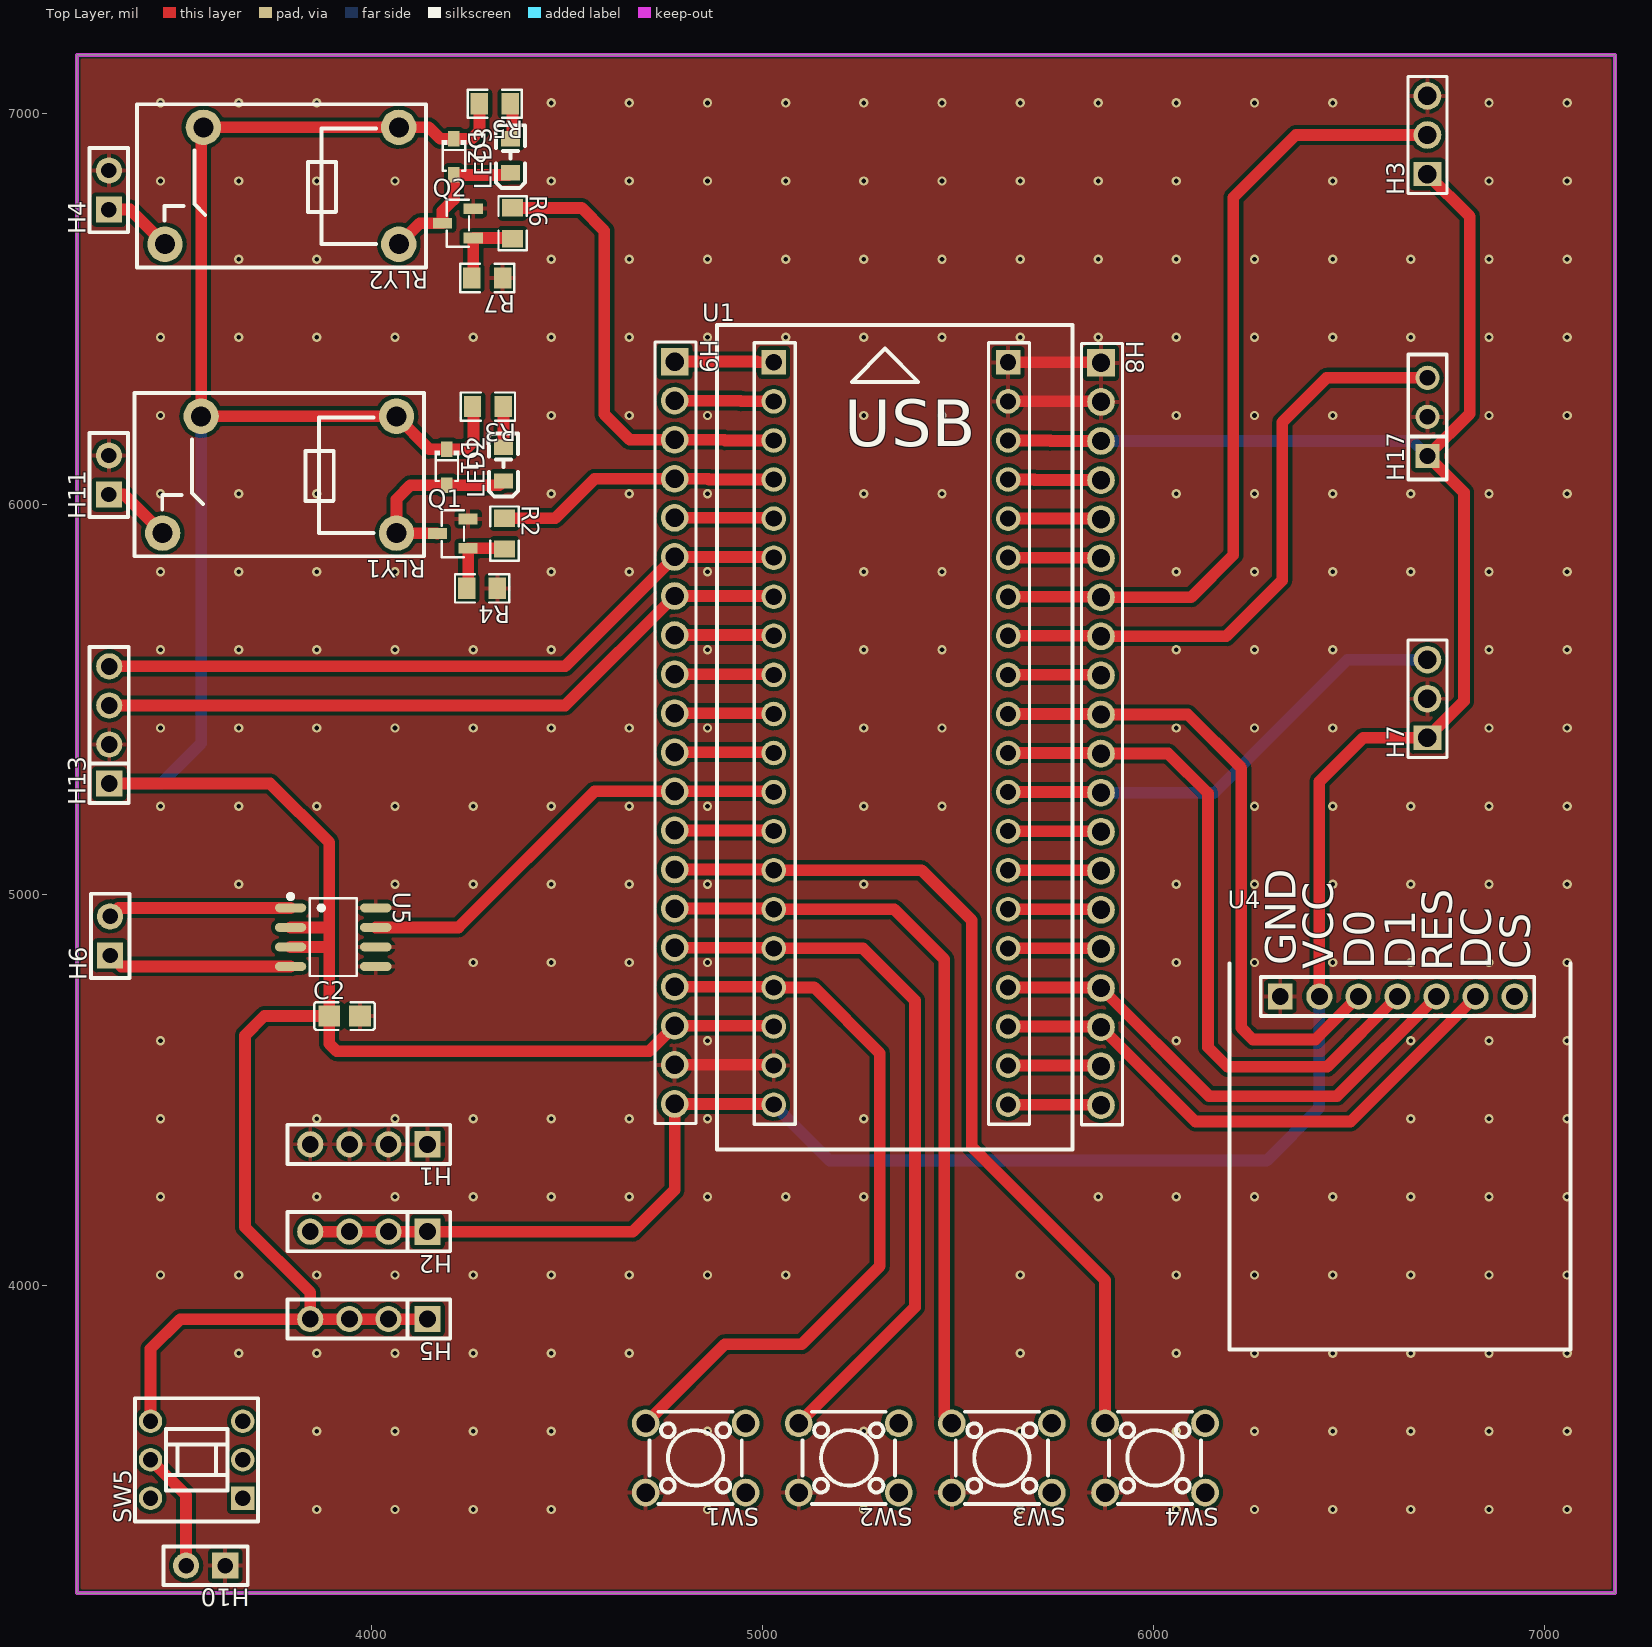
[diagram p0: Top Layer view]
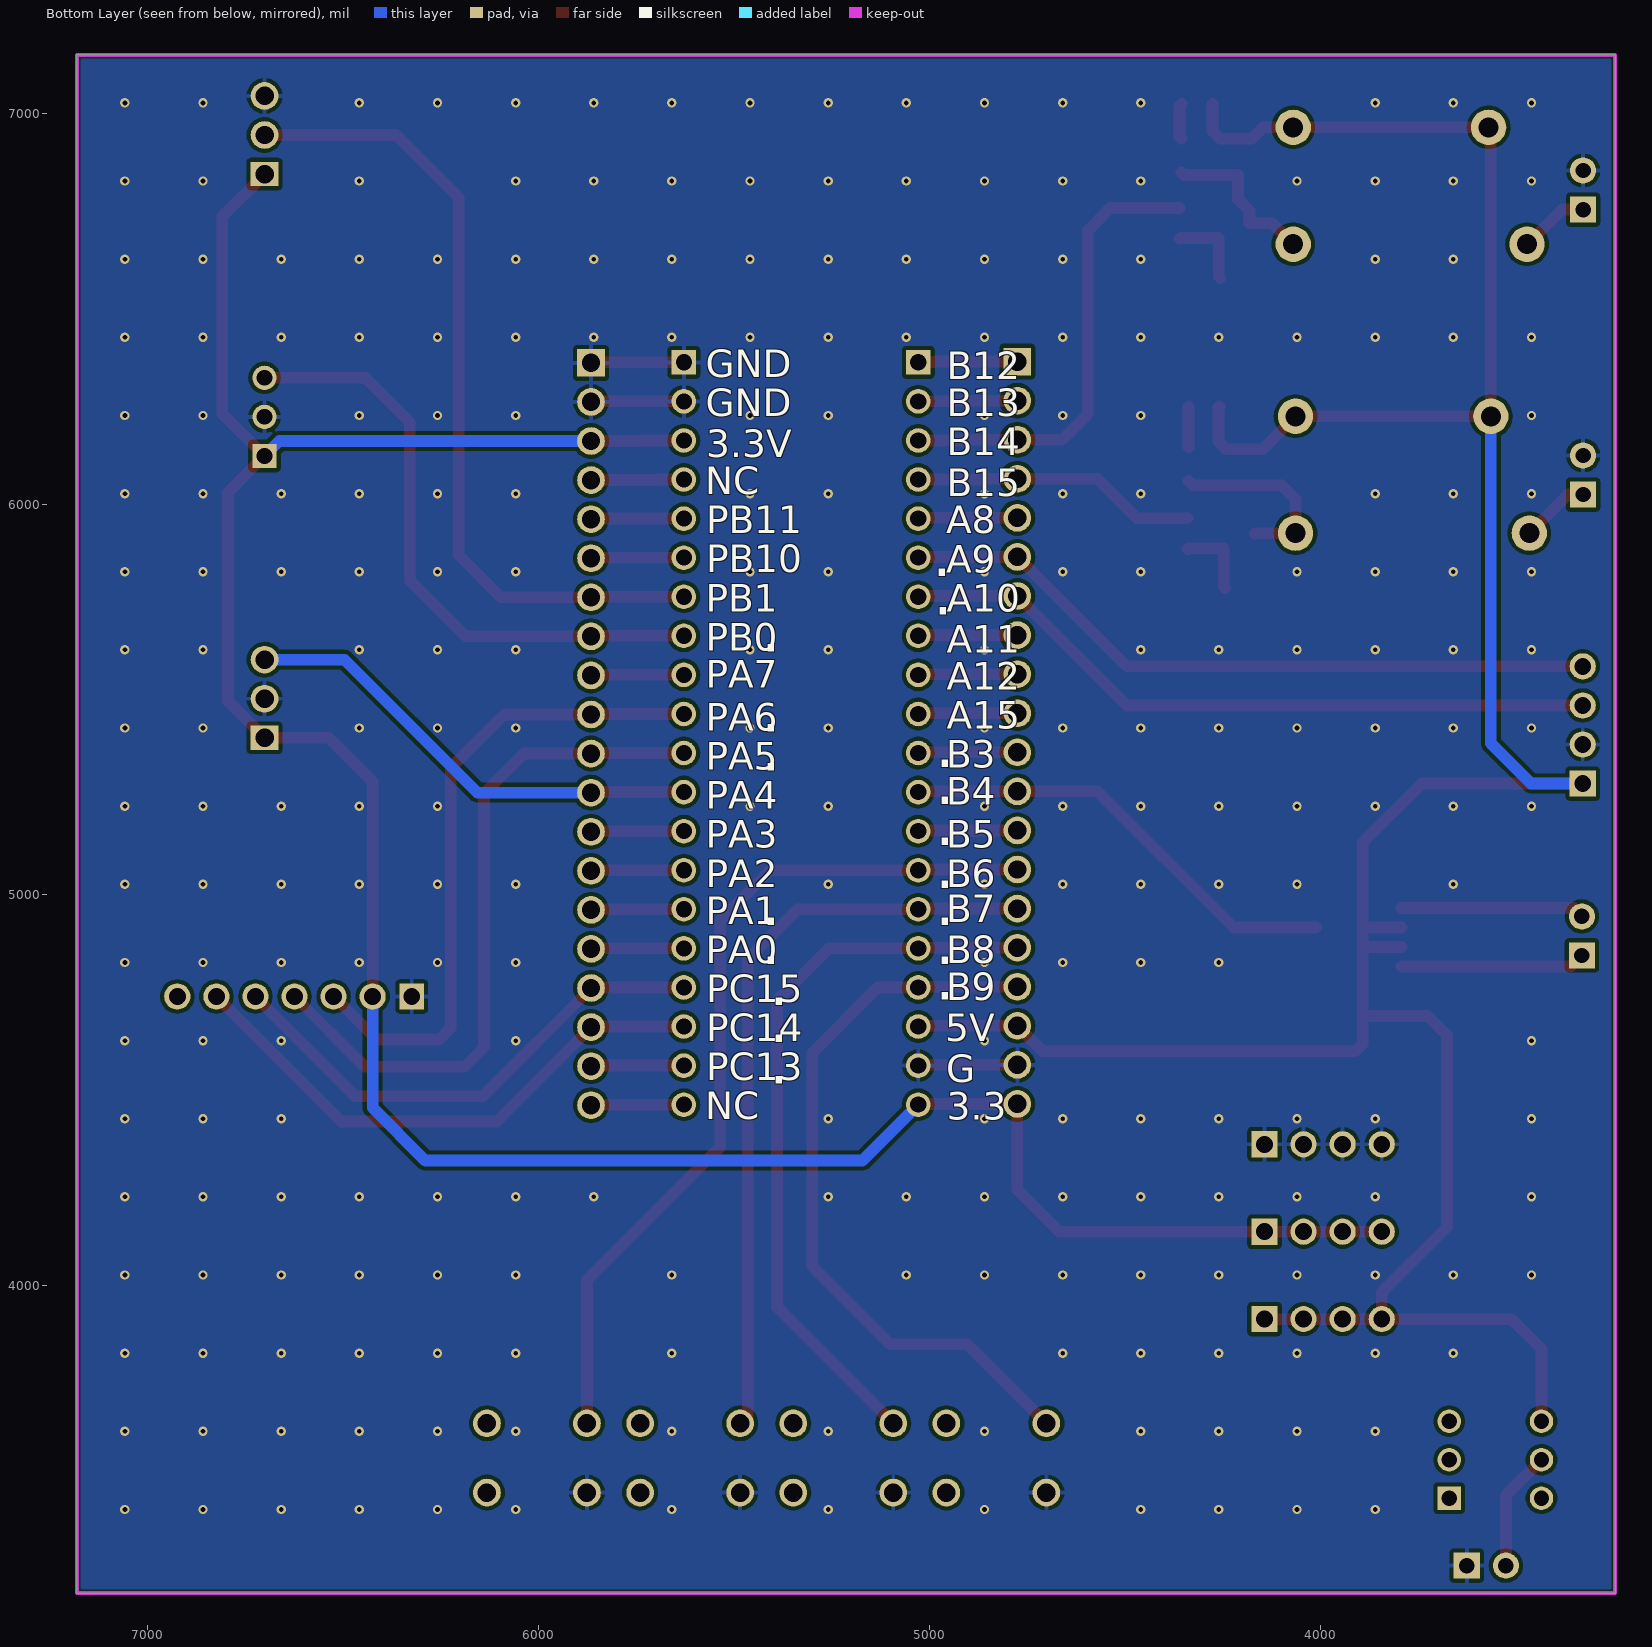
[diagram p1: Bottom Layer view, seen from below]
# Altium PCB MISC51992.pcbdoc
Units mil, origin at the board's own origin, x right, y up, seen from the top; angles counter-clockwise.
Board outline 3937.01 x 3937.01 mil, 2 copper layers (Top Layer, Bottom Layer), stack 62.206 mil thick; 36 components, 48 nets, 186 pads, 262 vias.

## Layer stack, top to bottom
Top Solder Mask Layer: solder mask 0.394, Dk 3.3
Top Layer: signal copper 1.379
Dielectric1: surface 59.449, FR4, Dk 4.5
Bottom Layer: signal copper 1.378
Bottom Solder Mask Layer: solder mask 0.394, Dk 3.3

## Board outline
3245,7150 3245,3212.99 7182.01,3212.99 7182.01,7150

## Design rules (kind name [scope] priority, off if disabled: settings)
BoardOutlineClearance copperThickness2oz_1 [All] p2 off: genericclearance=7.99 ignorepadtopadclearanceinfootprint=FALSE except(0: Arc-SplitContinuation Track-SplitContinuation SMDPad-SplitContinuation THPad-SplitContinuation Via-SplitContinuation Fill-SplitContinuation Region-SplitContinuation Poly-SplitContinuation Text-SplitContinuation Hole-SplitContinuation; 5.98: Arc-CutoutEdge SMDPad-CutoutEdge THPad-CutoutEdge Via-CutoutEdge Fill-CutoutEdge Region-CutoutEdge Text-CutoutEdge; 6.93: Hole-OutlineEdge Hole-CutoutEdge; 10: Poly-OutlineEdge Poly-CutoutEdge; 11.81: Arc-OutlineEdge Track-OutlineEdge SMDPad-OutlineEdge THPad-OutlineEdge Via-OutlineEdge Fill-OutlineEdge Region-OutlineEdge Text-OutlineEdge Track-CutoutEdge)
BoardOutlineClearance copperThickness1oz_1 [All] p4: genericclearance=4.02 ignorepadtopadclearanceinfootprint=FALSE except(0: Arc-SplitContinuation Track-SplitContinuation SMDPad-SplitContinuation THPad-SplitContinuation Via-SplitContinuation Fill-SplitContinuation Region-SplitContinuation Poly-SplitContinuation Text-SplitContinuation Hole-SplitContinuation; 6: SMDPad-CutoutEdge THPad-CutoutEdge Via-CutoutEdge Fill-CutoutEdge Region-CutoutEdge Text-CutoutEdge; 6.93: Hole-OutlineEdge Hole-CutoutEdge; 10: Poly-OutlineEdge Poly-CutoutEdge; 11.8: Arc-OutlineEdge Track-OutlineEdge SMDPad-OutlineEdge THPad-OutlineEdge Via-OutlineEdge Fill-OutlineEdge Region-OutlineEdge Text-OutlineEdge; 11.81: Arc-CutoutEdge Track-CutoutEdge)
Clearance copperThickness2oz [All] p1 off: gap=7.99 ignorepadtopadclearanceinfootprint=FALSE except(5.98: SMDPad-Track SMDPad-SMDPad THPad-Track SMDPad-THPad THPad-THPad Track-Via SMDPad-Via THPad-Via Via-Via Fill-Track Region-Track Fill-SMDPad Region-SMDPad Fill-THPad Region-THPad Fill-Via Region-Via Fill-Fill Fill-Region Region-Region Arc-Track Arc-SMDPad Arc-THPad Arc-Via Fill-Arc Region-Arc Arc-Arc Text-Track SMDPad-Text Text-THPad Text-Via Fill-Text Region-Text Arc-Text Text-Text; 6.93: Hole-Track Hole-SMDPad Hole-THPad Hole-Via Fill-Hole Region-Hole Hole-Arc Hole-Text; 10: Poly-Track Poly-SMDPad Poly-THPad Poly-Via Poly-Fill Poly-Region Poly-Poly Poly-Arc Poly-Text Poly-Hole)
Clearance copperThickness1oz [All] p3: gap=4.02 ignorepadtopadclearanceinfootprint=FALSE except(5.98: SMDPad-Track SMDPad-SMDPad THPad-Track SMDPad-THPad THPad-THPad Track-Via SMDPad-Via THPad-Via Via-Via Fill-Track Region-Track Fill-SMDPad Region-SMDPad Fill-THPad Region-THPad Fill-Via Region-Via Fill-Fill Fill-Region Region-Region; 6: Arc-Track Arc-SMDPad Arc-THPad Arc-Via Fill-Arc Region-Arc Arc-Arc Text-Track SMDPad-Text Text-THPad Text-Via Fill-Text Region-Text Arc-Text Text-Text; 6.93: Hole-Track Hole-SMDPad Hole-THPad Hole-Via Fill-Hole Region-Hole Hole-Arc Hole-Text; 10: Poly-Track Poly-SMDPad Poly-THPad Poly-Via Poly-Fill Poly-Region Poly-Poly Poly-Arc Poly-Text Poly-Hole)
DiffPairsRouting differentialPair [All] p1: maxlimit=6 minlimit=6 mostfreqgap=6 toplayer_minwidth=5 toplayer_prefwidth=10 toplayer_maxwidth=100 toplayer_mingap=6 toplayer_prefgap=6 toplayer_maxgap=6 bottomlayer_minwidth=5 bottomlayer_prefwidth=10 bottomlayer_maxwidth=100 bottomlayer_mingap=6 bottomlayer_prefgap=6 bottomlayer_maxgap=6 maxuncoupledlength=10
HoleToHoleClearance otherClearance [All] p1: gap=11.81 allowstackedmicrovias=TRUE
Length netLength [All] p1: minlimit=0 maxlimit=0
MatchedLengths netLengthTolerance [All] p1: tolerance=1000
PasteMaskExpansion pasteMaskExpansion [All] p1: expansion=0
PlaneConnect innerPlane [All] p1: planeconnectstyle=Relief reliefexpansion=20 reliefentries=4 reliefconductorwidth=10 reliefairgap=10
PolygonConnect copperRegion [(InNet('GND'))] p1: connectstyle=Relief reliefconductorwidth=10 reliefentries=4 polygonreliefangle="90 Angle" airgapwidth=10 via.connectstyle=Relief via.reliefconductorwidth=10 via.reliefentries=4 via.polygonreliefangle="90 Angle" via.airgapwidth=10
RoutingVias viaSize [All] p1: holewidth=12.01 width=24.02 viastyle="Through Hole" minholewidth=11.81 minwidth=19.68 maxholewidth=248.03 maxwidth=393.7
SolderMaskExpansion solderMaskExpansion [IsVia] p1: expansion=-1000 istentingtop=TRUE
SolderMaskExpansion solderMaskExpansion [All] p2: expansion=2 istentingtop=FALSE
Width copperThickness2oz_2 [All] p1 off: maxlimit=100 minlimit=8 preferedwidth=10
Width copperThickness1oz_2 [All] p2: maxlimit=100 minlimit=5 preferedwidth=10

## Components (designator, comment, footprint, x,y, rotation, side; value= is the part's Value field where it differs from the comment)
C2 "1uf" C0805 3930,4690 r0 top
D1 "1N4007WS" SOD-323_L1.8-W1.3-LS2.5-RD 4192.01,6094.72 r270 top
D2 "1N4007WS" SOD-323_L1.8-W1.3-LS2.5-RD 4210.11,6889 r270 top
H1 "" HDR-TH_4P-P2.54-V-F 3992.33,4361.73 r180 top
H2 "" HDR-TH_4P-P2.54-V-F 3992.33,4138.01 r180 top
H3 "Header-Male-2.54_1x3" HDR-TH_3P-P2.54-V-M-1 6701.59,6945 r90 top
H4 "" HDR-TH_2P-P2.54-V-F 3327.01,6804 r90 top
H5 "" HDR-TH_4P-P2.54-V-F 3992.33,3914.29 r180 top
H6 "" HDR-TH_2P-P2.54-V-F 3330,4895 r90 top
H7 "Header-Male-2.54_1x3" HDR-TH_3P-P2.54-V-M-1 6701.59,5502.04 r90 top
H8 "" HDR-TH_20P-P2.54-V-M-1 5866.11,5411.72 r270 top
H9 "" HDR-TH_20P-P2.54-V-M-1 4775,5415 r270 top
H10 "" HDR-TH_2P-P2.54-V-F 3574.54,3283.39 r180 top
H11 "" HDR-TH_2P-P2.54-V-F 3327.01,6074.72 r90 top
H13 "Header-Male-2.54_1x4" HDR-TH_4P-P2.54-V-M 3327.8,5435 r90 top
H17 "" HDR-TH_3P-P2.54-V-F 6701.81,6223.52 r90 top
LED2 "" LED_0805 4337.01,6104.72 r90 top
LED3 "" LED_0805 4355.11,6894 r90 top
Q1 "SS8050_C2150" SOT-23-3_L2.9-W1.3-P1.90-LS2.4-BR 4207.01,5924.72 r0 top
Q2 "SS8050_C2150" SOT-23-3_L2.9-W1.3-P1.90-LS2.4-BR 4220.11,6719 r0 top
R2 "4.7kΩ" R0805 4339.4,5924.81 r270 top
R3 "4.7kΩ" R0805 4297.01,6249.72 r180 top
R4 "10k" R0805 4282.01,5784.72 r180 top
R5 "4.7kΩ" R0805 4314.59,7025 r180 top
R6 "4.7kΩ" R0805 4360.11,6719 r270 top
R7 "10k" R0805 4295.11,6579 r180 top
RLY1 "JZC-32F/005-HS3(555)" RELAY-TH_JZC-32F-XXXHXX 3763.77,6075.44 r180 top
RLY2 "JZC-32F/005-HS3(555)" RELAY-TH_JZC-32F-XXXHXX 3769.59,6815 r180 top
SW1 "TS665CJ" SW-TH_4P-L6.0-W6.0-P4.50-LS6.5 4828.6,3558.98 r180 top
SW2 "TS665CJ" SW-TH_4P-L6.0-W6.0-P4.50-LS6.5 5220.56,3558.98 r180 top
SW3 "TS665CJ" SW-TH_4P-L6.0-W6.0-P4.50-LS6.5 5612.51,3558.98 r180 top
SW4 "TS665CJ" SW-TH_4P-L6.0-W6.0-P4.50-LS6.5 6004.47,3558.98 r180 top
SW5 "XKB8080-Z" SW-TH_6P-L8.0-W8.0-P2.50 3551.58,3554.25 r90 top
U1 "" STM32最小系统 5028.53,6363.15 r0 top
U4 "" OLED12864/7针 6325,4740 r0 top
U5 "L9110S_C2895059" SOP-8_L5.0-W4.0-P1.27-LS6.0-BL 3900.97,4891.78 r270 top

## Footprints (in the part's own frame and the unit in brackets; to place one, negate y for a bottom-side part, rotate by r counter-clockwise, add the part's x,y. Pads: shape width x height; smd on the part's side, far side on the other; paste and mask are expansions set on the pad)
C0805 [mm]
  rect 1.41x1.35 smd paste-100 mask+0.051: 1(-1,0) 2(1,0)
  silkscreen extent -1.96,-0.9 1.96,0.9
HDR-TH_2P-P2.54-V-F [mm]
  rect 1.7x1.7 hole 1: 1(-1.27,0)
  round 1.7 hole 1: 2(1.27,0)
  silkscreen extent -2.74,-1.25 2.74,1.25
HDR-TH_3P-P2.54-V-F [mil]
  rect 62x62 hole 40.16: 1(-100,0)
  round 62 hole 40.16: 2(0,0) 3(100,0)
  silkscreen extent -160,-49 160,49
HDR-TH_3P-P2.54-V-M-1 [mm]
  rect 1.575x1.8 hole 1.2: 1(-2.54,0)
  round 1.8 hole 1.2: 2(0,0) 3(2.54,0)
  silkscreen extent -3.81,-1.27 3.81,1.27
HDR-TH_4P-P2.54-V-F [mm]
  rect 1.7x1.7 hole 1.1: 1(-3.81,0)
  round 1.7 hole 1.1: 2(-1.27,0) 3(1.27,0) 4(3.81,0)
  silkscreen extent -5.29,-1.27 5.29,1.27
HDR-TH_4P-P2.54-V-M [mm]
  rect 1.7x1.7 hole 1.1: 1(-3.81,0)
  round 1.7 hole 1.1: 2(-1.27,0) 3(1.27,0) 4(3.81,0)
  silkscreen extent -5.08,-1.27 5.08,1.27
HDR-TH_20P-P2.54-V-M-1 [mm]
  rect 1.8x1.8 hole 1.2: 1(-24.13,0)
  round 1.8 hole 1.2: 2(-21.59,0) 3(-19.05,0) 4(-16.51,0) 5(-13.97,0) 6(-11.43,0) 7(-8.89,0) 8(-6.35,0) 9(-3.81,0) 10(-1.27,0) 11(1.27,0) 12(3.81,0) 13(6.35,0) 14(8.89,0) 15(11.43,0) 16(13.97,0) 17(16.51,0) 18(19.05,0) 19(21.59,0) 20(24.13,0)
  silkscreen extent -25.4,-1.27 25.4,1.4
LED_0805 [mm]
  rect 1x1.25 smd paste+0 mask+0.051: 1(-1.15,0.005) 2(1.05,0.005)
  silkscreen extent -2.15,-0.94 1.93,0.97
OLED12864/7针 [mm]
  rect 1.575x1.7 hole 1.1: 1(0,0)
  round 1.7 hole 1.1: 2(2.54,0) 3(5.08,0) 4(7.62,0) 5(10.16,0) 6(12.7,0) 7(15.24,0)
  silkscreen extent -3.3,-22.94 18.88,2.16
R0805 [mm]
  rect 1.133x1.377 smd paste-100 mask+0.051: 1(-1,0) 2(1,0)
  silkscreen extent -1.76,-0.92 1.76,0.92
RELAY-TH_JZC-32F-XXXHXX [mm]
  round 2.3 hole 1.3: 1(-7.6,-3.8) 2(-7.6,3.8) 3(7.6,3.8) 4(5.1,-3.8)
  silkscreen extent -9.38,-5.3 9.42,5.3
SOD-323_L1.8-W1.3-LS2.5-RD [mm]
  rect 1x0.75 smd: 1(-1.172,0) 2(1.172,0)
  silkscreen extent -1.08,-0.8 0.9,0.8
SOP-8_L5.0-W4.0-P1.27-LS6.0-BL [mil]
  oval 22.6x80.14 smd: 1(-75,-108.97) 2(-25,-108.97) 3(25,-108.97) 4(75,-108.97) 5(75,108.97) 6(25,108.97) 7(-25,108.97) 8(-75,108.97)
  silkscreen extent -110,-115 99,60
SOT-23-3_L2.9-W1.3-P1.90-LS2.4-BR [mm]
  rect 1.25x0.7 smd: 1(1,-0.95) 2(1,0.95) 3(-1,0)
  silkscreen extent -0.73,-1.53 0.73,1.53
STM32最小系统 [mm]
  rect 1.6x1.6 hole 1.05: 1(0,0) 21(15.24,0)
  round 1.6 hole 1.05: 2(0,-2.54) 3(0,-5.08) 4(0,-7.62) 5(0,-10.16) 6(0,-12.7) 7(0,-15.24) 8(0,-17.78) 9(0,-20.32) 10(0,-22.86) 11(0,-25.4) 12(0,-27.94) 13(0,-30.48) 14(0,-33.02) 15(0,-35.56) 16(0,-38.1) 17(0,-40.64) 18(0,-43.18) 19(0,-45.72) 20(0,-48.26) 22(15.24,-2.54) 23(15.24,-5.08) 24(15.24,-7.62) 25(15.24,-10.16) 26(15.24,-12.7) 27(15.24,-15.24) 28(15.24,-17.78) 29(15.24,-20.32) 30(15.24,-22.86) 31(15.24,-25.4) 32(15.24,-27.94) 33(15.24,-30.48) 34(15.24,-33.02) 35(15.24,-35.56) 36(15.24,-38.1) 37(15.24,-40.64) 38(15.24,-43.18) 39(15.24,-45.72) 40(15.24,-48.26)
  silkscreen extent -3.68,-51.18 19.43,2.41
SW-TH_4P-L6.0-W6.0-P4.50-LS6.5 [mm]
  round 1.8 hole 1.2: 1(-3.25,2.25) 2(3.25,2.25) 3(-3.25,-2.25) 4(3.25,-2.25)
  silkscreen extent -3,-3 3,3
SW-TH_6P-L8.0-W8.0-P2.50 [mm]
  rect 1.524x1.524 hole 1: 1(-2.5,-3)
  round 1.524 hole 1: 2(0,-3) 3(2.5,-3) 4(-2.5,3) 5(0,3) 6(2.5,3)
  silkscreen extent -4,-4 4,4

## Via types
v1: diameter 24.02, hole 12, Top Layer to Bottom Layer, 262 vias

## Nets (pads, with @x,y where several pads share a name; then routed paths per layer and width w, separated by ;. In a path a pad name is that pad's centre, name@x,y a point inside that pad or via, vN(x,y) a via of type N, cw(c..) or ccw(c..) an arc to the next point about the centre after c; other vN are vias at no path point)
3.3V: H2.1 H2.2 H2.3 H2.4 H3.1 H7.1 H8.3 H9.20 H17.1 U1.20 U1.23 U4.2 | length 6820.6
  Top Layer w30: H2.4 H2.3 H2.2 H2.1 4668.01,4138.01 4775,4245 H9.20 5026.68,4465 U1.20 ; U1.23 5736.4,6163.15 5737.84,6161.72 H8.3 ; U4.2 6425,5290 6537.04,5402.04 H7.1 6795,5495.44 6795,6030.32 H17.1 6810,6231.71 6810,6736.59 H3.1
  Bottom Layer w30: U1.20 5171.68,4320 6290,4320 6425,4455 U4.2 ; H8.3 6663.61,6161.72 H17.1
5V: C2.1 D1.1 D2.1 H5.1 H5.2 H5.3 H5.4 H9.18 H13.1 R3.2 R5.2 RLY1.1 RLY1.4 RLY2.1 RLY2.4 SW5.6 U1.18 U5.2 U5.3 | length 7952.6
  Top Layer w30: H13.1 3740,5285 3890.63,5134.37 3890.63,4916.78 ; SW5.6 3433.47,3838.47 3509.29,3914.29 H5.4 ; U5.3 3890.63,4866.78 ; U5.2 3890.63,4916.78 ; H5.1 H5.2 H5.3 H5.4 ; R3.2 4260,6247.35 4260,6160 4240.88,6140.88 D1.1 4147.15,6140.88 RLY1.1 RLY1.4 3562.98,6958.79 RLY2.4 RLY2.1 4145.4,6964.6 4174.84,6935.16 D2.1 4255.16,6935.16 4275.22,6955.22 R5.2 ; U1.18 5026.68,4665 H9.18 4710,4600 3910,4600 3890.63,4619.37 C2.1 ; H5.4 3842.33,3982.67 3675,4150 3675,4640 3725,4690 C2.1 ; C2.1 3890.63,4866.78 ; 3890.63,4866.78 3890.63,4916.78
  Bottom Layer w30: H13.1 3460,5285 3562.98,5387.98 RLY1.4
$1N1: H4.1 RLY2.3 | length 180.1
  Top Layer w30: H4.1 3381.78,6754 RLY2.3
$1N4: H11.1 RLY1.3 | length 178.5
  Top Layer w30: H11.1 3365.69,6024.72 RLY1.3
$1N7: H10.2 SW5.5 | length 308.6
  Top Layer w30: SW5.5 3524.54,3463.19 H10.2
$1N11: H6.1 U5.4 | length 473.7
  Top Layer w30: H6.1 3358.22,4816.78 U5.4
$1N12: H6.2 U5.1 | length 471
  Top Layer w30: H6.2 3351.78,4966.78 U5.1
$1N13: LED2.2 R3.1 | length 103.8
  Top Layer w30: R3.1 4336.81,6249.29 LED2.2
$1N14: LED3.2 R5.1 | length 94.3
  Top Layer w30: R5.1 4360,7018.96 4360,6940.43 LED3.2
$1N26: D1.2 LED2.1 Q1.3 RLY1.2 | length 485.3
  Top Layer w30: Q1.3 4166.51,5925.85 RLY1.2 4062.98,6012.98 4098.56,6048.56 D1.2 4325.93,6048.56 LED2.1
$1N27: D2.2 LED3.1 Q2.3 RLY2.2 | length 417.4
  Top Layer w30: RLY2.2 4122.39,6719 Q2.3 4180.74,6750.74 4210.11,6780.11 D2.2 4349.02,6842.84 LED3.1
$1N32: Q1.1 R2.2 R4.2 | length 197.9
  Top Layer w30: R4.2 4246.38,5788.46 Q1.1 4337.53,5887.32 R2.2
$1N33: Q2.1 R6.2 R7.2 | length 205.6
  Top Layer w30: R7.2 4259.48,6582.74 Q2.1 4358.14,6681.6 R6.2
$1N89: H8.4 U1.24 | length 238.2
  Top Layer w30: U1.24 5694.98,6063.15 5696.42,6061.72 H8.4
$1N90: H8.20 U1.40 | length 238.2
  Top Layer w30: U1.40 5864.68,4463.15 H8.20
GND: C2.2 H1.1 H1.2 H1.3 H1.4 H3.3 H4.2 H7.2 H8.1 H8.2 H9.19 H10.1 H11.2 H13.2 H17.2 Q1.2 Q2.2 R4.1 R7.1 SW1.2 SW2.2 SW3.2 SW4.2 U1.19 U1.21 U1.22 U4.1 U5.5 U5.6 U5.8 | length 730.7
  Top Layer w30: H9.19 5026.68,4565 U1.19 ; U1.22 5864.68,6263.15 H8.2 ; U1.21 5864.68,6363.15 H8.1
  other v1: 3859.1,3427.09 4059.1,3427.09 4259.1,3427.09 4459.1,3427.09 4859.1,3427.09 5259.1,3427.09 5659.1,3427.09 6059.1,3427.09 6259.1,3427.09 6459.1,3427.09 6659.1,3427.09 6859.1,3427.09 7059.1,3427.09 3859.1,3627.09 4059.1,3627.09 4259.1,3627.09 4459.1,3627.09 4859.1,3627.09 5259.1,3627.09 5659.1,3627.09 6059.1,3627.09 6259.1,3627.09 6459.1,3627.09 6659.1,3627.09 6859.1,3627.09 7059.1,3627.09 3659.1,3827.09 3859.1,3827.09 4059.1,3827.09 4259.1,3827.09 4459.1,3827.09 4659.1,3827.09 5659.1,3827.09 6059.1,3827.09 6259.1,3827.09 6459.1,3827.09 6659.1,3827.09 6859.1,3827.09 7059.1,3827.09 3459.1,4027.09 3659.1,4027.09 3859.1,4027.09 4059.1,4027.09 4259.1,4027.09 4459.1,4027.09 4659.1,4027.09 4859.1,4027.09 5059.1,4027.09 5659.1,4027.09 6059.1,4027.09 6259.1,4027.09 6459.1,4027.09 6659.1,4027.09 6859.1,4027.09 7059.1,4027.09 3459.1,4227.09 3859.1,4227.09 4059.1,4227.09 4259.1,4227.09 4459.1,4227.09 4659.1,4227.09 4859.1,4227.09 5059.1,4227.09 5259.1,4227.09 5859.1,4227.09 6059.1,4227.09 6259.1,4227.09 6459.1,4227.09 6659.1,4227.09 6859.1,4227.09 7059.1,4227.09 3459.1,4427.09 3859.1,4427.09 4059.1,4427.09 4259.1,4427.09 4459.1,4427.09 4659.1,4427.09 4859.1,4427.09 5259.1,4427.09 6659.1,4427.09 6859.1,4427.09 7059.1,4427.09 3459.1,4627.09 4859.1,4627.09 6059.1,4627.09 6659.1,4627.09 6859.1,4627.09 7059.1,4627.09 4259.1,4827.09 4459.1,4827.09 4659.1,4827.09 4859.1,4827.09 6059.1,4827.09 6259.1,4827.09 6459.1,4827.09 6659.1,4827.09 6859.1,4827.09 7059.1,4827.09 3659.1,5027.09 4059.1,5027.09 4259.1,5027.09 4459.1,5027.09 4659.1,5027.09 4859.1,5027.09 5259.1,5027.09 6059.1,5027.09 6259.1,5027.09 6459.1,5027.09 6659.1,5027.09 6859.1,5027.09 7059.1,5027.09 3459.1,5227.09 3659.1,5227.09 3859.1,5227.09 4059.1,5227.09 4259.1,5227.09 4459.1,5227.09 4659.1,5227.09 4859.1,5227.09 5259.1,5227.09 5459.1,5227.09 6259.1,5227.09 6459.1,5227.09 6659.1,5227.09 6859.1,5227.09 7059.1,5227.09 3459.1,5427.09 3659.1,5427.09 3859.1,5427.09 4059.1,5427.09 4259.1,5427.09 4459.1,5427.09 4659.1,5427.09 4859.1,5427.09 5259.1,5427.09 5459.1,5427.09 6059.1,5427.09 6259.1,5427.09 6459.1,5427.09 6859.1,5427.09 7059.1,5427.09 3459.1,5627.09 3659.1,5627.09 3859.1,5627.09 4059.1,5627.09 4259.1,5627.09 4459.1,5627.09 4859.1,5627.09 5259.1,5627.09 5459.1,5627.09 6059.1,5627.09 6259.1,5627.09 6459.1,5627.09 6859.1,5627.09 7059.1,5627.09 3459.1,5827.09 3659.1,5827.09 3859.1,5827.09 4059.1,5827.09 4459.1,5827.09 4659.1,5827.09 4859.1,5827.09 5259.1,5827.09 5459.1,5827.09 6059.1,5827.09 6259.1,5827.09 6459.1,5827.09 6659.1,5827.09 6859.1,5827.09 7059.1,5827.09 3459.1,6027.09 3659.1,6027.09 3859.1,6027.09 4459.1,6027.09 4659.1,6027.09 4859.1,6027.09 5259.1,6027.09 5459.1,6027.09 6059.1,6027.09 6259.1,6027.09 6459.1,6027.09 6659.1,6027.09 6859.1,6027.09 7059.1,6027.09 3459.1,6227.09 4459.1,6227.09 4659.1,6227.09 4859.1,6227.09 5259.1,6227.09 5459.1,6227.09 6059.1,6227.09 6259.1,6227.09 6459.1,6227.09 6859.1,6227.09 7059.1,6227.09 3459.1,6427.09 3659.1,6427.09 3859.1,6427.09 4059.1,6427.09 4259.1,6427.09 4459.1,6427.09 4659.1,6427.09 4859.1,6427.09 5059.1,6427.09 5259.1,6427.09 5459.1,6427.09 5659.1,6427.09 5859.1,6427.09 6059.1,6427.09 6259.1,6427.09 6459.1,6427.09 6659.1,6427.09 6859.1,6427.09 7059.1,6427.09 3659.1,6627.09 3859.1,6627.09 4459.1,6627.09 4659.1,6627.09 4859.1,6627.09 5059.1,6627.09 5259.1,6627.09 5459.1,6627.09 5659.1,6627.09 5859.1,6627.09 6059.1,6627.09 6259.1,6627.09 6459.1,6627.09 6659.1,6627.09 6859.1,6627.09 7059.1,6627.09 3459.1,6827.09 3659.1,6827.09 3859.1,6827.09 4059.1,6827.09 4459.1,6827.09 4659.1,6827.09 4859.1,6827.09 5059.1,6827.09 5259.1,6827.09 5459.1,6827.09 5659.1,6827.09 5859.1,6827.09 6059.1,6827.09 6459.1,6827.09 6859.1,6827.09 7059.1,6827.09 3459.1,7027.09 3659.1,7027.09 3859.1,7027.09 4459.1,7027.09 4659.1,7027.09 4859.1,7027.09 5059.1,7027.09 5259.1,7027.09 5459.1,7027.09 5659.1,7027.09 5859.1,7027.09 6059.1,7027.09 6259.1,7027.09 6459.1,7027.09 6859.1,7027.09 7059.1,7027.09
PA0: H8.16 U1.36 | length 238.2
  Top Layer w30: U1.36 5864.68,4863.15 H8.16
PA1: H8.15 U1.35 | length 238.2
  Top Layer w30: U1.35 5864.68,4963.15 H8.15
PA2: H8.14 U1.34 | length 238.2
  Top Layer w30: U1.34 5864.68,5063.15 H8.14
PA3: H8.13 U1.33 | length 238.2
  Top Layer w30: U1.33 5864.68,5163.15 H8.13
PA4: H7.3 H8.12 U1.32 | length 1214.6
  Top Layer w30: U1.32 5864.68,5263.15 H8.12
  Bottom Layer w30: H8.12 6156.72,5261.72 6497.04,5602.04 H7.3
PA5: H8.11 U1.31 U4.4 | length 1784.5
  Top Layer w30: U1.31 5864.68,5363.15 H8.11 6038.28,5361.72 6140,5260 6140,4610 6190,4560 6445,4560 U4.4
PA6: H8.10 U1.30 U4.3 | length 1676.7
  Top Layer w30: U1.30 5864.68,5463.15 H8.10 6088.28,5461.72 6225,5325 6225,4660 6255,4630 6415,4630 U4.3
PA7: H8.9 U1.29 | length 238.2
  Top Layer w30: U1.29 5864.68,5563.15 H8.9
PA8: H9.5 U1.5 | length 254.3
  Top Layer w30: H9.5 5026.68,5965 U1.5
PA9: H9.6 H13.4 U1.6 | length 1817.5
  Top Layer w30: H13.4 4495,5585 H9.6 5026.68,5865 U1.6
PA10: H9.7 H13.3 U1.7 | length 1817.5
  Top Layer w30: H13.3 4495,5485 H9.7 5026.68,5765 U1.7
PA11: H9.8 U1.8 | length 254.3
  Top Layer w30: H9.8 5026.68,5665 U1.8
PA12: H9.9 U1.9 | length 254.3
  Top Layer w30: H9.9 5026.68,5565 U1.9
PA15: H9.10 U1.10 | length 254.3
  Top Layer w30: H9.10 5026.68,5465 U1.10
PB0: H8.8 H17.3 U1.28 | length 1585.2
  Top Layer w30: U1.28 5864.68,5663.15 H8.8 6186.72,5661.72 6330,5805 6330,6210 6443.52,6323.52 H17.3
PB1: H3.2 H8.7 U1.27 | length 2099.8
  Top Layer w30: U1.27 5864.68,5763.15 H8.7 6096.72,5761.72 6205,5870 6205,6785 6365,6945 H3.2
PB3: H9.11 U1.11 | length 254.3
  Top Layer w30: H9.11 5026.68,5365 U1.11
PB4: H9.12 U1.12 U5.7 | length 1163.6
  Top Layer w30: U5.7 4221.78,4916.78 4570,5265 H9.12 5026.68,5265 U1.12
PB5: H9.13 U1.13 | length 254.3
  Top Layer w30: H9.13 5026.68,5165 U1.13
PB6: H9.14 SW4.4 U1.14 | length 2242.8
  Top Layer w30: H9.14 5026.68,5065 U1.14 5406.85,5063.15 5535,4935 5535,4355 5876.52,4013.48 SW4.4
PB7: H9.15 SW3.4 U1.15 | length 1939.4
  Top Layer w30: H9.15 5026.68,4965 U1.15 5336.85,4963.15 5465,4835 5465,3667.12 SW3.4
PB8: H9.16 SW2.4 U1.16 | length 1876.5
  Top Layer w30: H9.16 5026.68,4865 U1.16 5256.85,4863.15 5390,4730 5390,3944.95 SW2.4
PB9: H9.17 SW1.4 U1.17 | length 1906.5
  Top Layer w30: SW1.4 4903.1,3850 5100,3850 5300,4050 5300,4595 5131.85,4763.15 U1.17 5026.68,4765 H9.17
PB10: H8.6 U1.26 | length 238.2
  Top Layer w30: U1.26 5864.68,5863.15 H8.6
PB11: H8.5 U1.25 | length 238.2
  Top Layer w30: U1.25 5864.68,5963.15 H8.5
PB12: H9.1 U1.1 | length 254.3
  Top Layer w30: H9.1 4985.18,6365 4987.03,6363.15 U1.1
PB13: H9.2 U1.2 | length 254.3
  Top Layer w30: H9.2 4943.76,6265 4945.61,6263.15 U1.2
PB14: H9.3 R6.1 U1.3 | length 1190.3
  Top Layer w30: R6.1 4536.63,6758.37 4595,6700 4595,6230 4660,6165 H9.3 4902.34,6165 4904.19,6163.15 U1.3
PB15: H9.4 R2.1 U1.4 | length 731.6
  Top Layer w30: R2.1 4469.19,5964.19 4570,6065 H9.4 4860.92,6065 4862.77,6063.15 U1.4
PC13: H8.19 U1.39 | length 238.2
  Top Layer w30: U1.39 5864.68,4563.15 H8.19
PC14: H8.18 U1.38 U4.6 | length 1429.7
  Top Layer w30: U1.38 5864.68,4663.15 H8.18 6107.83,4420 6505,4420 U4.6
PC15: H8.17 U1.37 U4.5 | length 1317.3
  Top Layer w30: U1.37 5864.68,4763.15 H8.17 6142.83,4485 6470,4485 U4.5
pads on no net: SW1.1 SW1.3 SW2.1 SW2.3 SW3.1 SW3.3 SW4.1 SW4.3 SW5.1 SW5.2 SW5.3 SW5.4 U4.7

## Polygon pours and split planes (outlines as drawn)
GND on Top Layer (solid, remove dead copper, pour order 0): 3000,7300 3000,3000 7465,3000 7465,7300
GND on Bottom Layer (solid, remove dead copper, pour order 2): 3055,7195 3055,3095 7245,3095 7245,7195

## Keep-outs
Board Outline Layer:
  the board outline again, w10